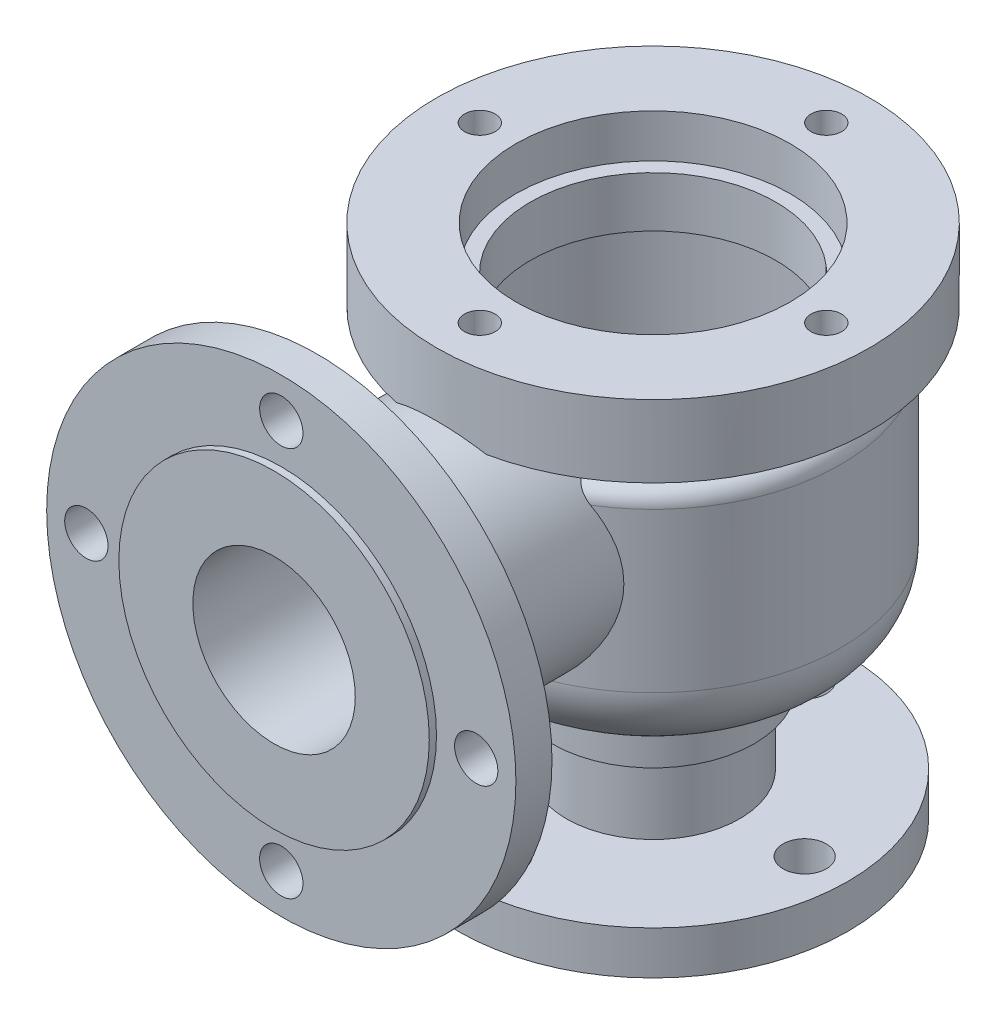
SolidWorks part; units mm, degrees
ref_plane "Front Plane" through (0, 0, 0) normal (0, 0, 1) x (1, 0, 0)
ref_plane "Top Plane" through (0, 0, 0) normal (0, 1, 0) x (1, 0, 0)
ref_plane "Right Plane" through (0, 0, 0) normal (1, 0, 0) x (0, 0, -1)
other "Configuration Table"
sketch "Sketch1" plane through (0, 0, 0) normal (1, 0, 0) x (0, 0, -1)
  line L0 (0, 101.241) -> (0, -76.9816) construction
  line L1 (0, 0) -> (32, 0)
  line L2 (32, 0) -> (32, 2)
  line L3 (32, 2) -> (54, 2)
  line L4 (54, 2) -> (54, 14)
  line L5 (54, 14) -> (24, 14)
  line L6 (24, 14) -> (24, 34)
  line L7 (24, 34) -> (28, 34)
  line L8 (28, 34) -> (28, 46)
  line L9 (31, 49) -> (32, 49)
  line L10 (52, 69) -> (52, 113)
  line L13 (48, 125) -> (60, 125)
  line L14 (60, 125) -> (60, 145)
  line L15 (60, 145) -> (0, 145)
  line L16 (0, 145) -> (0, 0)
  arc A2 (47, 118) -> (52, 113) centre (47, 113) cw
  arc A3 (48, 125) -> (44, 121) centre (48, 121) ccw
  arc A4 (44, 121) -> (47, 118) centre (47, 121) ccw
  arc A5 (32, 49) -> (52, 69) centre (32, 69) ccw
  arc A6 (28, 46) -> (31, 49) centre (31, 46) cw
  dimension "D14" = 88
  dimension "D6" = 5
  dimension "D15" = 4
  dimension "D16" = 3
  dimension "D17" = 20
  dimension "D18" = 3
  dimension "D1" = 64
  dimension "D2" = 108
  dimension "D3" = 48
  dimension "D4" = 56
  dimension "D5" = 104
  dimension "D7" = 120
  dimension "D8" = 20
  dimension "D9" = 2
  dimension "D10" = 12
  dimension "D11" = 34
  dimension "D12" = 15
  dimension "D13" = 145
revolve "Revolve1" add sketch "Sketch1" angle 360 about L0
sketch "Sketch2" plane through (0, 0, 0) normal (1, 0, 0) x (0, 0, -1)
  line L0 (-163.3124, 95) -> (59.6757, 95) construction
  line L1 (-105, 117.5) -> (-105, 138)
  line L2 (-105, 138) -> (-103, 138)
  line L3 (-103, 138) -> (-103, 160)
  line L4 (-103, 160) -> (-93, 160)
  line L5 (-93, 160) -> (-93, 127.5)
  line L6 (-93, 127.5) -> (-37.3968, 127.5)
  line L7 (-37.3968, 127.5) -> (-37.3968, 95)
  line L8 (-105, 117.5) -> (-41.5741, 117.5)
  line L9 (-41.5741, 117.5) -> (-41.5741, 95)
  line L10 (-41.5741, 95) -> (-37.3968, 95)
  dimension "D1" = 95
  dimension "D2" = 45
  dimension "D3" = 65
  dimension "D4" = 130
  dimension "D5" = 86
  dimension "D6" = 2
  dimension "D7" = 10
  dimension "D8" = 105
revolve "Revolve2" add sketch "Sketch2" angle 360 about L0
sketch "Sketch3" plane through (0, 0, 105) normal (0, 0, 1) x (1, 0, 0)
  line L0 (-15.8193, 111) -> (15.8193, 111)
  circle A0 centre (0, 95) radius 22.5
  circle M2 centre (0, 95) radius 22.5
  dimension "D1" = 45
  dimension "D2" = 16
extrude "Cut-Extrude1" cut sketch "Sketch3" against normal blind 120 contours L0 M2
sketch "Sketch4" plane through (0, 0, 0) normal (1, 0, 0) x (0, 0, -1)
  line L0 (0, 158.3481) -> (0, -5.3598) construction
  line L1 (0, 145) -> (38, 145)
  line L2 (60, 145) -> (-60, 145) construction
  line L3 (38, 145) -> (38, 133)
  line L4 (38, 133) -> (34, 133)
  line L5 (34, 133) -> (34, 119)
  line L6 (34, 119) -> (38.85, 119)
  line L7 (38.85, 119) -> (46, 113.0004)
  line L8 (46, 113.0004) -> (46, 69)
  line L9 (32, 55) -> (26, 55)
  line L10 (26, 55) -> (26, 63)
  line L11 (26, 63) -> (22, 63)
  line L12 (22, 63) -> (22, 45)
  line L13 (22, 45) -> (18, 45)
  line L14 (18, 45) -> (18, 0)
  line L15 (-32, 0) -> (32, 0) construction
  line L16 (18, 0) -> (0, 0)
  line L17 (0, 0) -> (0, 145)
  line L18 (-31, 49) -> (31, 49) construction
  arc A0 (46, 69) -> (32, 55) centre (32, 69) cw
  dimension "D14" = 14
  dimension "D1" = 12
  dimension "D2" = 76
  dimension "D3" = 77.7
  dimension "D4" = 50
  dimension "D5" = 26
  dimension "D6" = 68
  dimension "D7" = 92
  dimension "D8" = 44
  dimension "D9" = 52
  dimension "D10" = 36
  dimension "D11" = 18
  dimension "D12" = 63
  dimension "D13" = 6
revolve "Cut-Revolve1" cut sketch "Sketch4" angle 360 about L0
sketch "Sketch5" plane through (0, 0, 103) normal (0, 0, 1) x (1, 0, 0)
  circle A0 centre (0, 95) radius 54 construction
  circle A1 centre (0, 149) radius 6
  circle A2 centre (54, 95) radius 6
  circle A3 centre (0, 41) radius 6
  circle A4 centre (-54, 95) radius 6
  point P14 (0, 95)
  dimension "D1" = 108
  dimension "D2" = 12
  dimension "D3" = 4
extrude "Cut-Extrude2" cut sketch "Sketch5" against normal up to next
sketch "Sketch6" plane through (0, 2, 0) normal (0, -1, 0) x (1, 0, 0)
  circle A0 centre (0, 0) radius 42 construction
  circle A1 centre (42, 0) radius 6
  circle A2 centre (0, -42) radius 6
  circle A3 centre (-42, 0) radius 6
  circle A4 centre (0, 42) radius 6
  point P14 (0, 0)
  dimension "D1" = 84
  dimension "D2" = 12
  dimension "D3" = 4
extrude "Cut-Extrude3" cut sketch "Sketch6" against normal up to next
sketch "Sketch7" plane through (0, 145, 0) normal (0, 1, 0) x (1, 0, 0)
  circle A0 centre (0, 0) radius 48 construction
  circle A1 centre (0, 48) radius 6
  circle A2 centre (48, 0) radius 6
  circle A3 centre (0, -48) radius 6
  circle A4 centre (-48, 0) radius 6
  point P3 (0, 48)
  point P8 (48, 0)
  point P10 (0, -48)
  point P12 (-48, 0)
  point P14 (0, 0)
  dimension "D1" = 96
  dimension "D2" = 12
  dimension "D3" = 4
hole_wizard "M10 Tapped Hole1" positions "Sketch7" profile "Sketch8" tap size "M10" standard "GB"
sketch "Sketch8" plane through (0, 145, 0) normal (1, 0, 0) x (0, 0, 1)
  line L0 (0, 0) -> (0, 27.0537)
  line L1 (0, 27.0537) -> (4.25, 24.5)
  line L2 (4.25, 24.5) -> (4.25, 0)
  line L5 (4.25, 0) -> (0, 0)
  line L10 (0, 27.0537) -> (-4.25, 24.5) construction
  line L11 (0, -6.35) -> (0, 107.95) construction
  dimension "螺纹孔钻头直径" = 8.5
  dimension "螺纹孔钻头深度" = 24.5
  dimension "导头角度" = 118
cosmetic thread "Cosmetic Thread 1" parameters "D1"=20, "D2"=10
cosmetic thread "Cosmetic Thread 2" parameters "D1"=20, "D2"=10
cosmetic thread "Cosmetic Thread 3" parameters "D1"=20, "D2"=10
cosmetic thread "Cosmetic Thread 4" parameters "D1"=20, "D2"=10
sketch "Sketch9" plane through (0, 0, 0) normal (0, 0, 1) x (1, 0, 0)
  circle A0 centre (0, 76) radius 3
  circle A1 centre (0, 106) radius 3
  point P0 (0, 76)
  point P2 (0, 106)
  dimension "D1" = 76
  dimension "D3" = 6
  dimension "D4" = 6
  dimension "D2" = 30
hole_wizard "M6 Tapped Hole1" positions "Sketch9" profile "Sketch11" tap size "M6" standard "GB"
sketch "Sketch11" plane through (0, 76, 0) normal (1, 0, 0) x (0, -1, 0)
  line L0 (0, 0) -> (0, 60)
  line L1 (0, 60) -> (2.5, 60)
  line L2 (2.5, 60) -> (2.5, 0)
  line L5 (2.5, 0) -> (0, 0)
  line L11 (0, -6.35) -> (0, 107.95) construction
  dimension "通孔螺纹孔钻头直径" = 5
  dimension "通孔螺纹孔钻头深度" = 60
cosmetic thread "Cosmetic Thread 5" parameters "D2"=6
cosmetic thread "Cosmetic Thread 6" parameters "D2"=6
